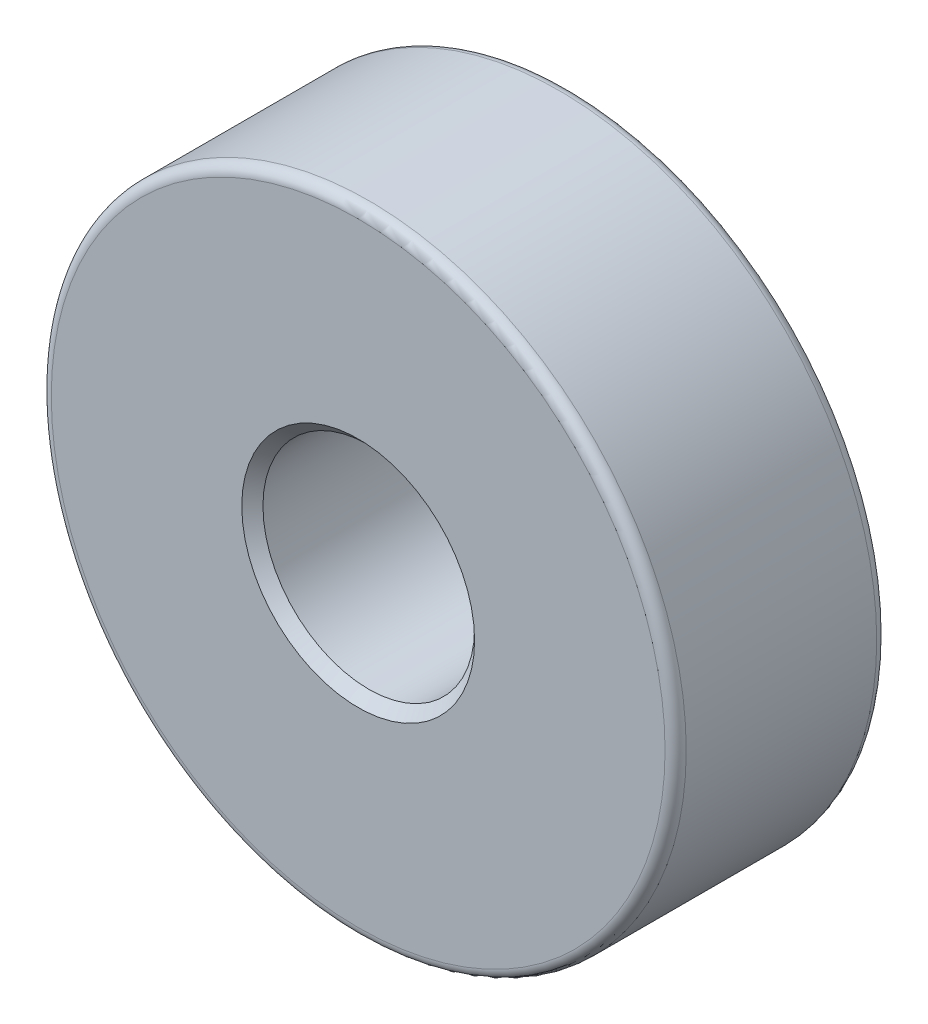
SolidWorks part; units mm, degrees
material "35"
ref_plane "前视基准面" through (0, 0, 0) normal (0, 0, 1) x (1, 0, 0)
ref_plane "上视基准面" through (0, 0, 0) normal (0, 1, 0) x (1, 0, 0)
ref_plane "右视基准面" through (0, 0, 0) normal (1, 0, 0) x (0, 0, -1)
sketch "草图1" plane through (0, 0, 0) normal (0, 0, 1) x (1, 0, 0)
  circle A0 centre (0, 0) radius 5
  circle A1 centre (0, 0) radius 15
  dimension "D1" = 10
  dimension "D2" = 30
extrude "凸台-拉伸1" add sketch "草图1" along normal blind 10
fillet "圆角1" radius 0.5 2 edges at (15, 0, 0) (15, 0, 10)
chamfer "倒角1" distance 0.5 angle 45 2 edges at (5, 0, 0) (5, 0, 10)
